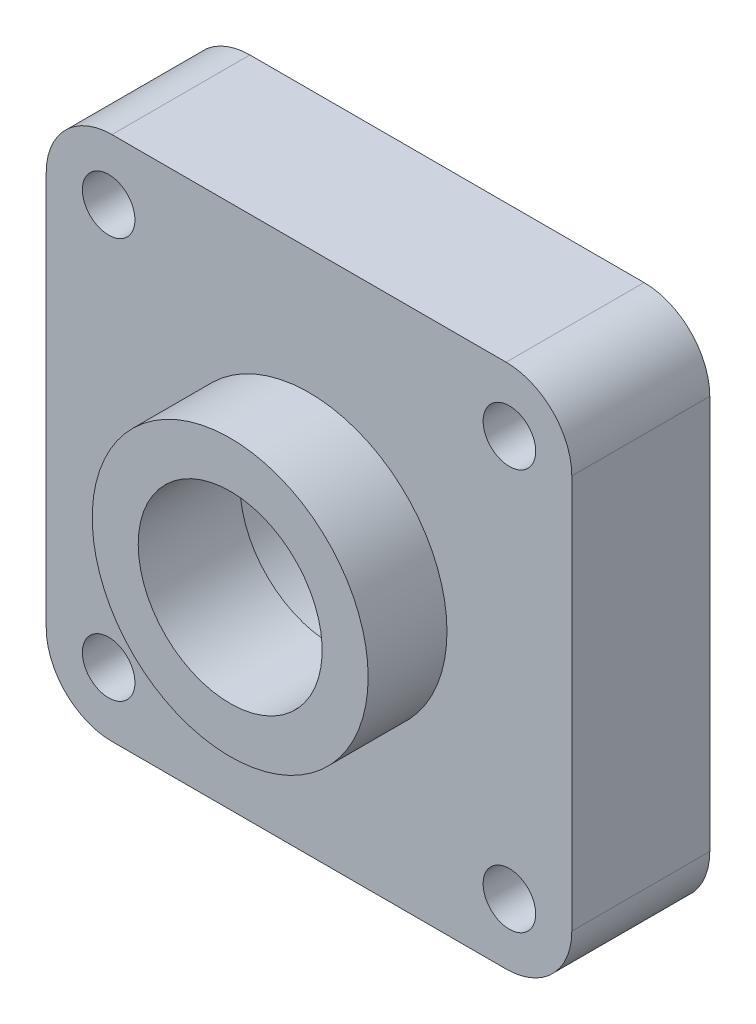
SolidWorks part; units mm, degrees
material "ZSnSb7Cu4"
ref_plane "前视基准面" through (0, 0, 0) normal (0, 0, 1) x (1, 0, 0)
ref_plane "上视基准面" through (0, 0, 0) normal (0, 1, 0) x (1, 0, 0)
ref_plane "右视基准面" through (0, 0, 0) normal (1, 0, 0) x (0, 0, -1)
sketch "草图1" plane through (0, 0, 0) normal (0, 0, 1) x (1, 0, 0)
  line L1 (-40, -40) -> (40, -40)
  line L2 (-40, -40) -> (-40, 40)
  line L3 (-40, 40) -> (40, 40)
  line L4 (40, -40) -> (40, 40)
  line L5 (-40, -40) -> (40, 40) construction
  line L6 (-40, 40) -> (40, -40) construction
  point P0 (0, 0)
  dimension "D1" = 80
  dimension "D2" = 80
extrude "凸台-拉伸1" add sketch "草图1" along normal blind 21
sketch "草图2" plane through (0, 0, 21) normal (0, 0, 1) x (1, 0, 0)
  circle A0 centre (0, 0) radius 21
  dimension "D1" = 42
extrude "凸台-拉伸2" add sketch "草图2" along normal blind 12
sketch "草图3" plane through (0, 0, 0) normal (0, 1, 0) x (1, 0, 0)
  line L0 (0, 0) -> (0, -32.0177) construction
  line L1 (30, 0) -> (30, -2.5)
  line L2 (40, 0) -> (-40, 0) construction
  line L3 (30, -2.5) -> (22.5, -2.5)
  line L4 (22.5, -2.5) -> (22.5, -7.5)
  line L5 (22.5, -7.5) -> (17.5, -7.5)
  line L6 (17.5, -7.5) -> (17.5, -15.5)
  line L7 (17.5, -15.5) -> (20, -15.5)
  line L8 (20, -15.5) -> (20, -17.5)
  line L9 (20, -17.5) -> (14, -17.5)
  line L10 (14, -17.5) -> (14, -33)
  line L11 (-21, -33) -> (21, -33) construction
  line L12 (30, 0) -> (0, 0)
  line L13 (0, 0) -> (0, -33)
  line L14 (0, -33) -> (14, -33)
  point P7 (0, -16.0089)
  dimension "D1" = 30
  dimension "D2" = 2.5
  dimension "D3" = 45
  dimension "D4" = 35
  dimension "D5" = 20
  dimension "D6" = 28
  dimension "D7" = 8
  dimension "D8" = 5
  dimension "D9" = 2
revolve "切除-旋转1" cut sketch "草图3" angle 360 about L0
sketch "草图4" plane through (0, 0, 21) normal (0, 0, 1) x (1, 0, 0)
  line L0 (-40, 40) -> (-14.8492, 14.8492) construction
  circle A0 centre (0, 0) radius 21 construction
fillet "圆角1" radius 10 4 edges at (40, -40, 10.5) (-40, -40, 10.5) (40, 40, 10.5) (-40, 40, 10.5)
sketch "草图6" plane through (0, 0, 21) normal (0, 0, 1) x (1, 0, 0)
  line L0 (-40, 40) -> (-14.8492, 14.8492) construction
  line L1 (-40, 30) -> (-40, -30) construction
  circle A0 centre (-30.5, 30.5) radius 4
  dimension "D1" = 8
  dimension "D2" = 9.5
extrude "切除-拉伸1" cut sketch "草图6" against normal blind 21
mirror "镜向1" about plane through (0, 0, 0) normal (0, 1, 0) of "切除-拉伸1"
mirror "镜向2" about plane through (0, 0, 0) normal (1, 0, 0) of "镜向1", "切除-拉伸1"
fillet "圆角2" radius 1 1 edges at (-30, 0, 2.5)
fillet "圆角3" radius 1 1 edges at (-20, 0, 17.5)
